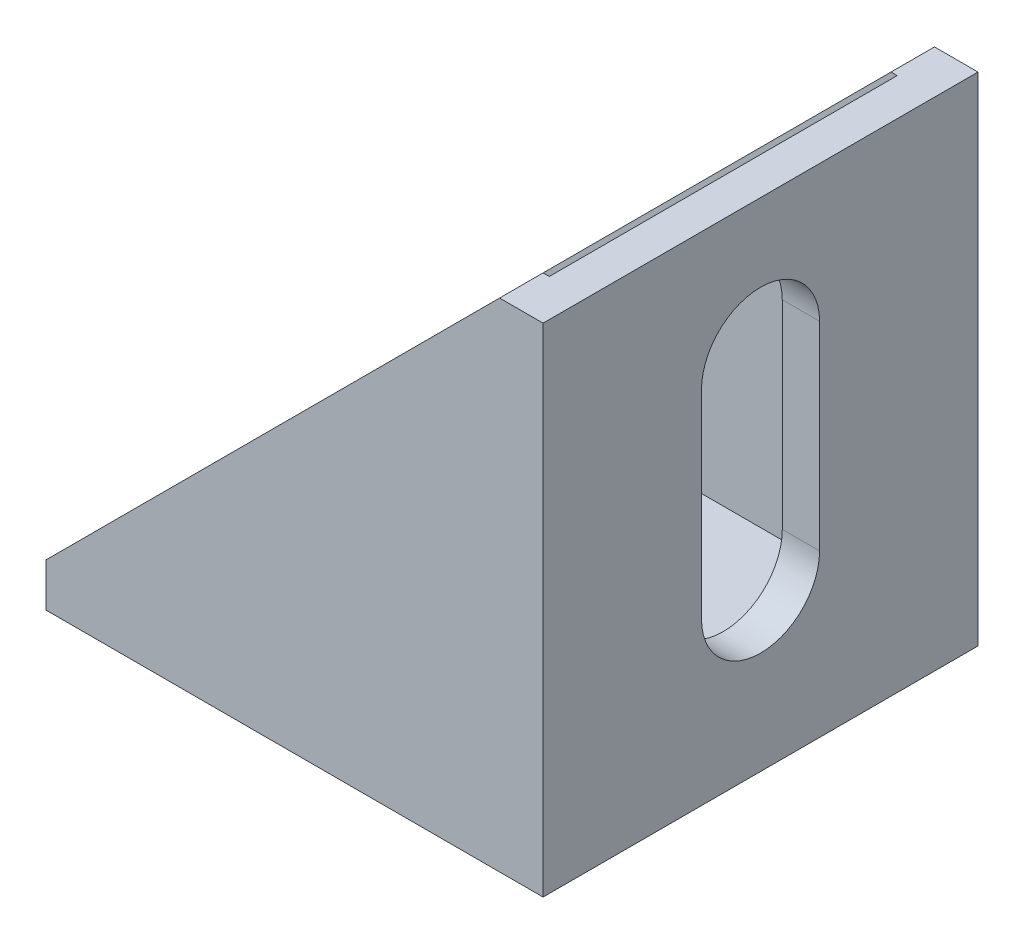
SolidWorks part; units mm, degrees
ref_plane "主视基准图" through (0, 0, 0) normal (0, 0, 1) x (1, 0, 0)
ref_plane "上视基准图" through (0, 0, 0) normal (0, 1, 0) x (1, 0, 0)
ref_plane "右视基准图" through (0, 0, 0) normal (1, 0, 0) x (0, 0, -1)
sketch "草图1" plane through (0, 0, 0) normal (0, 0, 1) x (1, 0, 0)
  line L0 (-22.5, 0) -> (-22.5, 3.5)
  line L1 (-22.5, 0) -> (17.5, 0)
  line L2 (17.5, 40) -> (14, 40)
  line L3 (14, 40) -> (-22.5, 3.5)
  line L4 (17.5, 0) -> (17.5, 40)
  dimension "D1" = 40
  dimension "D2" = 40
  dimension "D3" = 3.5
  dimension "D4" = 3.5
extrude "凸台-拉伸1" add sketch "草图1" along normal mid plane 35
sketch "草图2" plane through (0, 0, 0) normal (0, 0, 1) x (1, 0, 0)
  line L0 (14.5, 3) -> (14.5, 49.2902)
  line L1 (14.5, 36.2574) -> (14.5, 36.2574)
  line L3 (-18.7574, 3) -> (-18.7574, 3)
  line L4 (-34.1951, 3) -> (14.5, 3)
  line L5 (17.5, 0) -> (17.5, 40)
  line L6 (17.5, 40) -> (14, 40)
  line L7 (14, 40) -> (-22.5, 3.5)
  line L8 (-22.5, 3.5) -> (-22.5, 0)
  line L9 (-22.5, 0) -> (17.5, 0)
  line L10 (17.5, 0) -> (17.5, 40) construction
  line L11 (17.5, 40) -> (14, 40) construction
  line L12 (14, 40) -> (-22.5, 3.5) construction
  line L13 (-22.5, 3.5) -> (-22.5, 0) construction
  line L14 (-22.5, 0) -> (17.5, 0) construction
  line L15 (-18.7574, 3) -> (14.5, 3) construction
  line L17 (14.5, 3) -> (14.5, 36.2574) construction
  line L18 (14.5, 49.2902) -> (-34.1951, 3)
  line L20 (14.5, 36.2574) -> (-18.7574, 3) construction
  dimension "D1" = 0
  dimension "D2" = 3
extrude "切除-拉伸1" cut sketch "草图2" along normal mid plane 28 contours L18 L4 L0
sketch "草图4" plane through (0, 3, 0) normal (0, 1, 0) x (1, 0, 0)
  line L0 (-11.5, 0) -> (4.5, 0) construction
  line L1 (-11.5, 4.75) -> (4.5, 4.75)
  line L2 (-11.5, -4.75) -> (4.5, -4.75)
  line L5 (-22.5, 14) -> (-22.5, -14) construction
  arc A0 (-11.5, 4.75) -> (-11.5, -4.75) centre (-11.5, 0) ccw
  arc A1 (4.5, -4.75) -> (4.5, 4.75) centre (4.5, 0) ccw
  point P3 (-3.5, 0)
  dimension "D3" = 11
  dimension "D1" = 16
  dimension "D2" = 9.5
extrude "切除-拉伸2" cut sketch "草图4" against normal through all
sketch "草图5" plane through (14.5, 0, 0) normal (-1, 0, 0) x (0, 0, 1)
  line L0 (0, 13) -> (0, 29) construction
  line L1 (-4.75, 13) -> (-4.75, 29)
  line L2 (4.75, 13) -> (4.75, 29)
  line L5 (14, 40) -> (-14, 40) construction
  arc A0 (-4.75, 13) -> (4.75, 13) centre (0, 13) ccw
  arc A1 (4.75, 29) -> (-4.75, 29) centre (0, 29) ccw
  point P2 (0, 21)
  dimension "D3" = 11
  dimension "D1" = 16
  dimension "D2" = 9.5
extrude "切除-拉伸3" cut sketch "草图5" against normal through all
ref_plane "基准面1" through (0, 0, 0) normal (0, 0, 1) x (1, 0, 0)
ref_plane "基准面2" through (0, 0, 0) normal (0, 0, 1) x (1, 0, 0)
